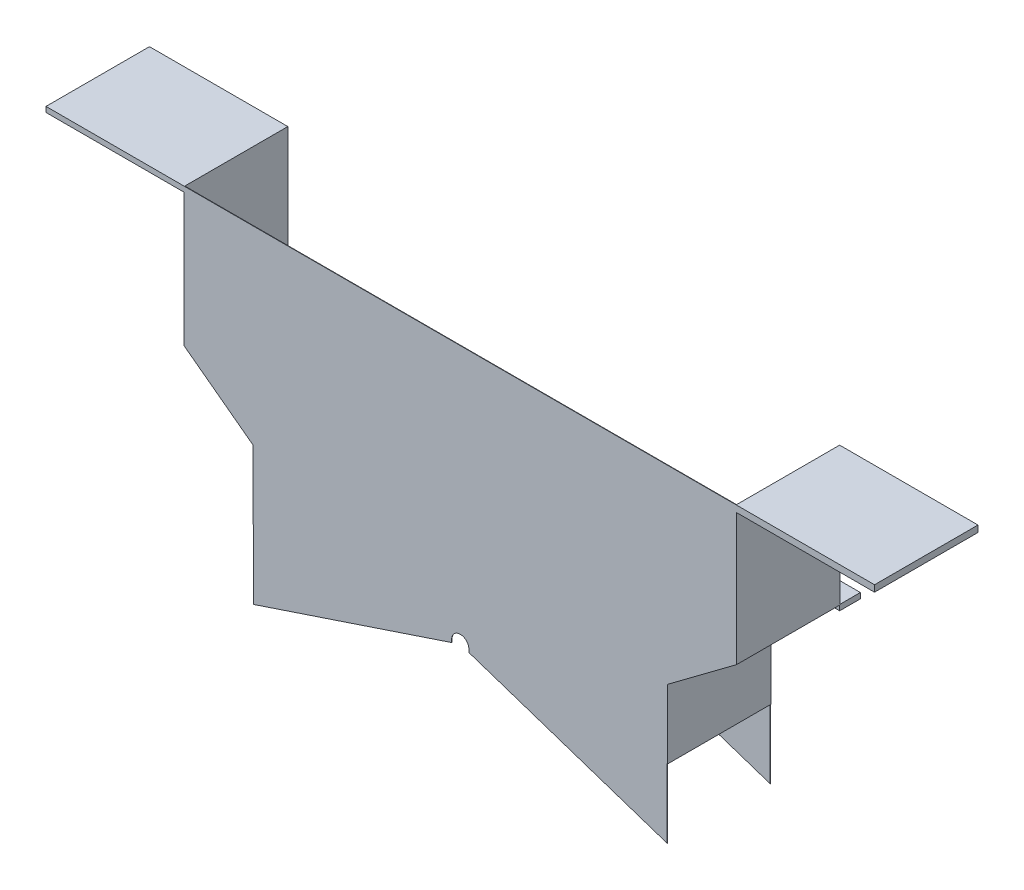
SolidWorks part; units mm, degrees
ref_plane "前视基准面" through (0, 0, 0) normal (0, 0, 1) x (1, 0, 0)
ref_plane "上视基准面" through (0, 0, 0) normal (0, 1, 0) x (1, 0, 0)
ref_plane "右视基准面" through (0, 0, 0) normal (1, 0, 0) x (0, 0, -1)
sketch "草图1" plane through (0, 0, 0) normal (0, 0, 1) x (1, 0, 0)
  line L0 (0, 1143.7674) -> (0, 100) construction
  line L1 (0, 0) -> (-50000, 0) construction
  line L2 (0, 90) -> (0, -81.7456) construction
  line L3 (300, 0) -> (300, 230)
  line L4 (300, 230) -> (-300, 230)
  line L5 (-300, 230) -> (-300, 0)
  line L7 (-9.4868, 96.8377) -> (-300, 0)
  line L8 (9.4868, 96.8377) -> (300, 0)
  arc A0 (9.4868, 96.8377) -> (-9.4868, 96.8377) centre (0, 100) ccw
  dimension "D1" = 230
extrude "凸台-拉伸1" add sketch "草图1" along normal blind 0.6
sketch "草图4" plane through (0, 0, 0) normal (0, 0, -1) x (-1, 0, 0)
  line L0 (-400, 375) -> (-400, 275)
  line L1 (300, 100) -> (300.6, 100)
  line L2 (300, 100) -> (300, 200)
  line L3 (0, 0) -> (0, 275.48) construction
  line L4 (300.6, 100) -> (300.6, 200)
  line L6 (-400.6003, 274.6995) -> (-400.6003, 375)
  line L7 (-400.6003, 375) -> (-400, 375)
  line L8 (400.6003, 274.6995) -> (300.6, 200)
  line L9 (0, 100) -> (412.3868, 100) construction
  line L10 (400, 275) -> (300, 200.3007)
  line L11 (300, 200) -> (300, 200.3007)
  line L12 (-300, 200) -> (-300, 200.3007)
  line L13 (-400, 275) -> (-300, 200.3007)
  line L14 (-400.6003, 274.6995) -> (-300.6, 200)
  line L15 (-300.6, 100) -> (-300.6, 200)
  line L16 (-300, 100) -> (-300, 200)
  line L17 (400.6003, 375) -> (400, 375)
  line L18 (-300, 100) -> (-300.6, 100)
  line L19 (400.6003, 274.6995) -> (400.6003, 375)
  line L20 (400, 375) -> (400, 275)
  line L21 (300, 230) -> (300, 0) construction
  dimension "D1" = 0
  dimension "D2" = 100
  dimension "D3" = 100
  dimension "D4" = 0.6
  dimension "D5" = 0
  dimension "D6" = 0.6
  dimension "D7" = 100
  dimension "D8" = 75
  dimension "D9" = 0.6003
  dimension "D10" = 100
extrude "凸台-拉伸2" add sketch "草图4" against normal blind 150
sketch "草图5" plane through (0, 0, 150) normal (0, 0, 1) x (1, 0, 0)
  line L0 (-300, 0) -> (-300, 100)
  line L1 (-400.6003, 274.6995) -> (-400.6003, 375) construction
  line L4 (-300, 100) -> (-300.6, 100)
  line L5 (-300.6, 100) -> (-300.6, 200)
  line L6 (-300.6, 200) -> (-400.6003, 274.6995)
  line L7 (-400.6003, 274.6995) -> (-400.6003, 375)
  line L8 (-400.6003, 375) -> (400.6003, 375)
  line L9 (400.6003, 375) -> (400.6003, 274.6995)
  line L10 (400.6003, 274.6995) -> (300.6, 200)
  line L11 (300.6, 200) -> (300.6, 115)
  line L12 (300.6, 115) -> (300, 115)
  line L13 (300, 115) -> (300, 0)
  line L14 (300, 0) -> (9.4868, 96.8377)
  line L15 (-9.4868, 96.8377) -> (-300, 0)
  arc A0 (9.4868, 96.8377) -> (-9.4868, 96.8377) centre (0, 100) ccw
extrude "凸台-拉伸3" add sketch "草图5" against normal blind 0.6
sketch "草图6" plane through (0, 0, 0) normal (0, 0, -1) x (-1, 0, 0)
  line L0 (-300, 230) -> (-340.6, 230)
  line L1 (-300, 230) -> (300, 230) construction
  line L2 (-300, 200.3007) -> (-300, 230) construction
  line L4 (-340.6, 230) -> (-300.6, 200)
  line L5 (-300, 200.3) -> (-300, 230)
  line L6 (300, 230) -> (343.6518, 232.1594)
  line L7 (300.6, 200) -> (400.6003, 274.6995) construction
  line L8 (343.6518, 232.1594) -> (300.6, 200)
  line L9 (300.6, 200) -> (300, 200.3007)
  line L10 (300, 200.3007) -> (300, 230)
  arc A0 (-300.6, 200) -> (-300, 200.3) centre (-300.375, 200.3) ccw
extrude "凸台-拉伸4" add sketch "草图6" against normal blind 0.6
sketch "草图7" plane through (0, 0, 150) normal (0, 0, 1) x (1, 0, 0)
  line L0 (-12.5, 100) -> (-12.5, 86.1037)
  line L1 (-12.5, 86.1037) -> (12.5, 86.1037)
  line L2 (12.5, 86.1037) -> (12.5, 100)
  arc A0 (12.5, 100) -> (-12.5, 100) centre (0, 100) ccw
extrude "切除-拉伸1" cut sketch "草图7" against normal through all
sketch "草图8" plane through (0, 375, 0) normal (0, 1, 0) x (1, 0, 0)
  line L0 (-400.6003, -150) -> (400.6003, -150) construction
  line L1 (-400.6003, 0) -> (-400, 0)
  line L2 (-400.6003, 0) -> (-400.6003, -150)
  line L3 (-400.6003, -150) -> (-400, -150)
  line L4 (-400, 0) -> (-400, -149.4)
  line L5 (400.6003, -150) -> (400.6003, 0) construction
  line L6 (-400, -150) -> (400.6003, -150)
  line L8 (-400, -149.4) -> (400, -149.4)
  line L9 (400.6003, -150) -> (400.6003, -149.4)
  line L12 (400.6003, -149.4) -> (400.6003, 0)
  line L13 (400.6003, 0) -> (400, 0)
  line L14 (400, -149.4) -> (400, 0)
extrude "凸台-拉伸5" add sketch "草图8" along normal blind 100
sketch "草图9" plane through (-400.6003, 0, 0) normal (-1, 0, 0) x (0, 0, 1)
  line L0 (0, 475) -> (150, 475)
  line L1 (150, 475) -> (150, 467.3166)
  line L2 (150, 274.6995) -> (150, 475) construction
  line L3 (150, 467.3166) -> (0, 467.3166)
  line L4 (0, 274.6995) -> (0, 475) construction
  line L5 (0, 467.3166) -> (0, 475)
extrude "凸台-拉伸6" add sketch "草图9" along normal blind 200
sketch "草图11" plane through (400.6003, 0, 0) normal (1, 0, 0) x (0, 0, -1)
  line L0 (-150, 475) -> (0, 475)
  line L1 (0, 475) -> (0, 465.5991)
  line L2 (0, 475) -> (0, 274.6995) construction
  line L3 (0, 465.5991) -> (-150, 465.5991)
  line L4 (-150, 475) -> (-150, 274.6995) construction
  line L5 (-150, 465.5991) -> (-150, 475)
extrude "凸台-拉伸7" add sketch "草图11" along normal blind 200
sketch "草图12" plane through (0, 0, 0) normal (0, 0, -1) x (-1, 0, 0)
  line L0 (-339.7585, 230) -> (-400, 275)
  line L1 (-400, 275) -> (400.6003, 274.6995)
  line L2 (400.6003, 274.6995) -> (342.5782, 232.1063)
  line L3 (342.5782, 232.1063) -> (-339.7585, 230)
extrude "凸台-拉伸10" add sketch "草图12" against normal blind 2
ref_plane "基准面1" through (-0.1032, 274.8498, 0) normal (-0.0004, 1, 0) x (1, 0.0004, 0)
sketch "草图16" plane through (-0.1032, 274.8498, 0) normal (-0.0004, 1, 0) x (1, 0.0004, 0)
  line L0 (-399.8217, 0) -> (-399.8217, 30)
  line L1 (-399.8217, 30) -> (400.1782, 30)
  line L2 (400.1782, 30) -> (400.1782, 0)
  line L3 (400.1782, 0) -> (-399.8217, 0)
  dimension "D1" = 30
extrude "凸台-拉伸12" add sketch "草图16" against normal blind 8
